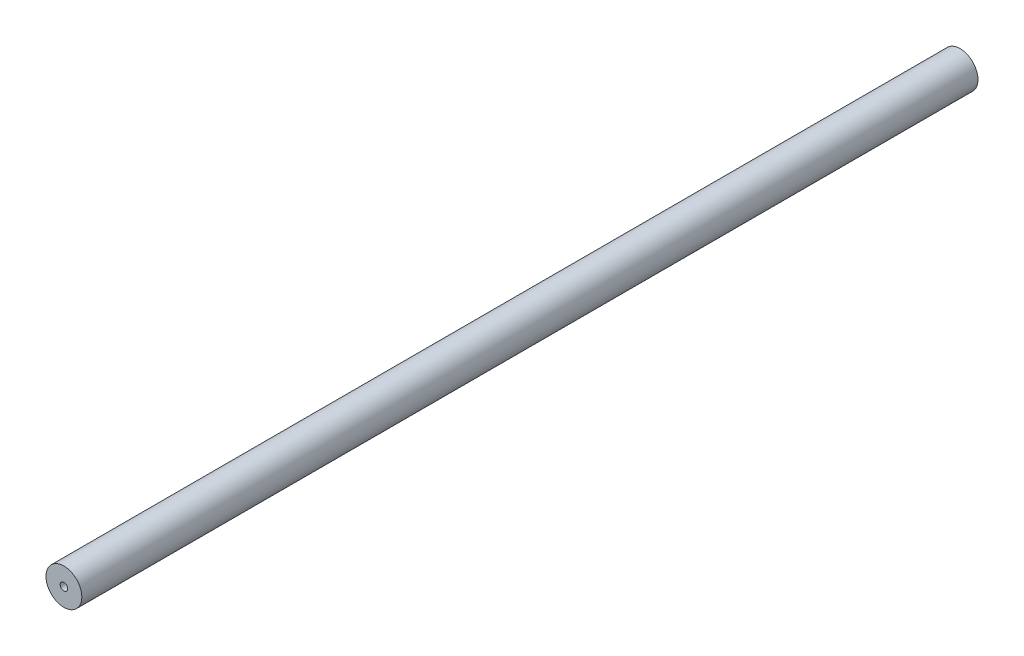
SolidWorks part; units mm, degrees
ref_plane "前视基准面" through (0, 0, 0) normal (0, 0, 1) x (1, 0, 0)
ref_plane "上视基准面" through (0, 0, 0) normal (0, 1, 0) x (1, 0, 0)
ref_plane "右视基准面" through (0, 0, 0) normal (1, 0, 0) x (0, 0, -1)
sketch "草图1" plane through (0, 0, 0) normal (0, 0, 1) x (1, 0, 0)
  circle A0 centre (0, 0) radius 10
  dimension "D1" = 20
extrude "凸台-拉伸1" add sketch "草图1" along normal blind 500
hole_wizard "M5 螺纹孔1" positions "草图4" profile "草图3" tap size "M5" standard "Iso"
sketch "草图4" plane through (0, 0, 0) normal (0, 0, -1) x (-1, 0, 0)
  point P0 (0, 0)
sketch "草图3" plane through (0, 0, 0) normal (1, 0, 0) x (0, 1, 0)
  line L0 (0, 0) -> (0, 13.6618)
  line L1 (0, 13.6618) -> (2.1, 12.4)
  line L2 (2.1, 12.4) -> (2.1, 0)
  line L5 (2.1, 0) -> (0, 0)
  line L10 (0, 13.6618) -> (-2.1, 12.4) construction
  line L11 (0, -6.35) -> (0, 107.95) construction
  dimension "螺纹孔钻头直径" = 4.2
  dimension "螺纹孔钻头深度" = 12.4
  dimension "导头角度" = 118
cosmetic thread "孔螺蚊线1" parameters "D1"=10, "D2"=5
hole_wizard "M5 螺纹孔2" positions "草图6" profile "草图5" tap size "M5" standard "Iso"
sketch "草图6" plane through (0, 0, 500) normal (0, 0, 1) x (1, 0, 0)
  point P0 (0, 0)
sketch "草图5" plane through (0, 0, 500) normal (1, 0, 0) x (0, -1, 0)
  line L0 (0, 0) -> (0, 13.6618)
  line L1 (0, 13.6618) -> (2.1, 12.4)
  line L2 (2.1, 12.4) -> (2.1, 0)
  line L5 (2.1, 0) -> (0, 0)
  line L10 (0, 13.6618) -> (-2.1, 12.4) construction
  line L11 (0, -6.35) -> (0, 107.95) construction
  dimension "螺纹孔钻头直径" = 4.2
  dimension "螺纹孔钻头深度" = 12.4
  dimension "导头角度" = 118
cosmetic thread "孔螺蚊线2"
